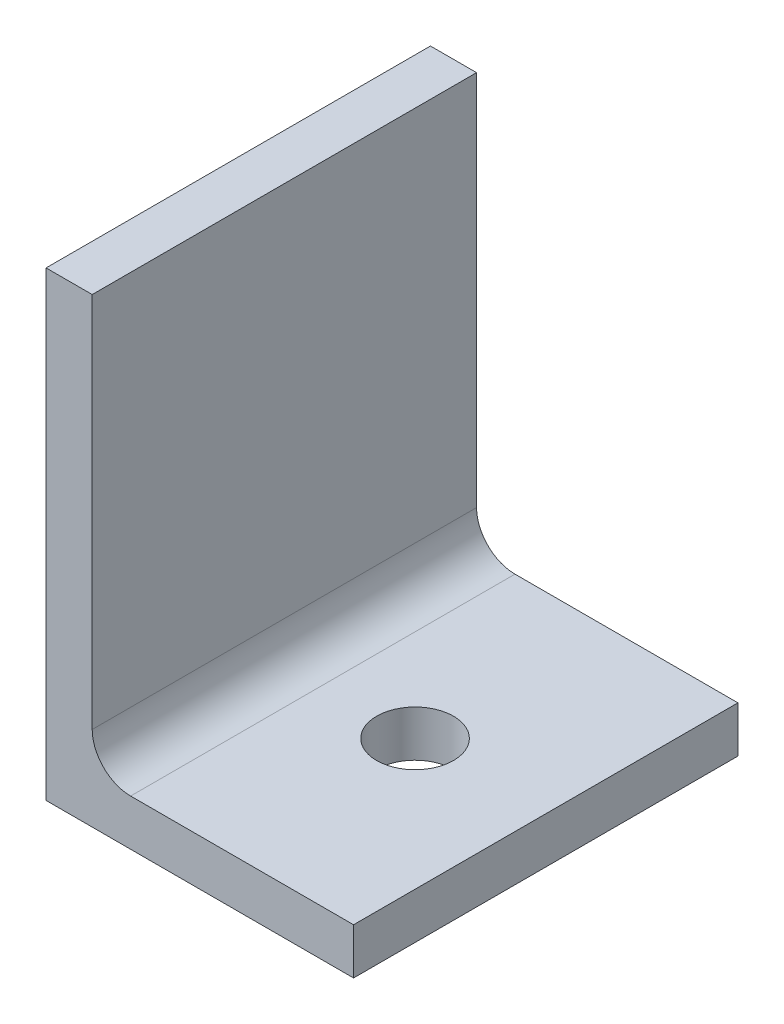
SolidWorks part; units mm, degrees
material "1023 碳钢板 (SS)"
ref_plane "Front Plane" through (0, 0, 0) normal (0, 0, 1) x (1, 0, 0)
ref_plane "Top Plane" through (0, 0, 0) normal (0, 1, 0) x (1, 0, 0)
ref_plane "Right Plane" through (0, 0, 0) normal (1, 0, 0) x (0, 0, -1)
sketch "Sketch1" plane through (0, 0, 0) normal (0, 0, 1) x (1, 0, 0)
  line L0 (0, 0) -> (0, -120)
  line L1 (0, -120) -> (80, -120)
  line L2 (12, 0) -> (12, -98)
  line L3 (22, -108) -> (80, -108)
  line L4 (12, 0) -> (12, -108) construction
  line L5 (12, -108) -> (80, -108) construction
  line L6 (12, 0) -> (0, 0)
  line L7 (80, -108) -> (80, -120)
  arc A0 (12, -98) -> (22, -108) centre (22, -98) ccw
  dimension "D4" = 10
  dimension "D1" = 80
  dimension "D2" = 120
  dimension "D3" = 12
extrude "Boss-Extrude1" add sketch "Sketch1" along normal blind 100 contours L7 L1 L0 L6 L2 A0 L3
sketch "Sketch2" plane through (0, -108, 0) normal (0, 1, 0) x (1, 0, 0)
  line L0 (80, -100) -> (80, 0) construction
  circle A0 centre (46, -50) radius 10
  point P5 (80, -50)
  dimension "D1" = 34
  dimension "D2" = 20
extrude "Cut-Extrude1" cut sketch "Sketch2" against normal blind 100 contours A0
